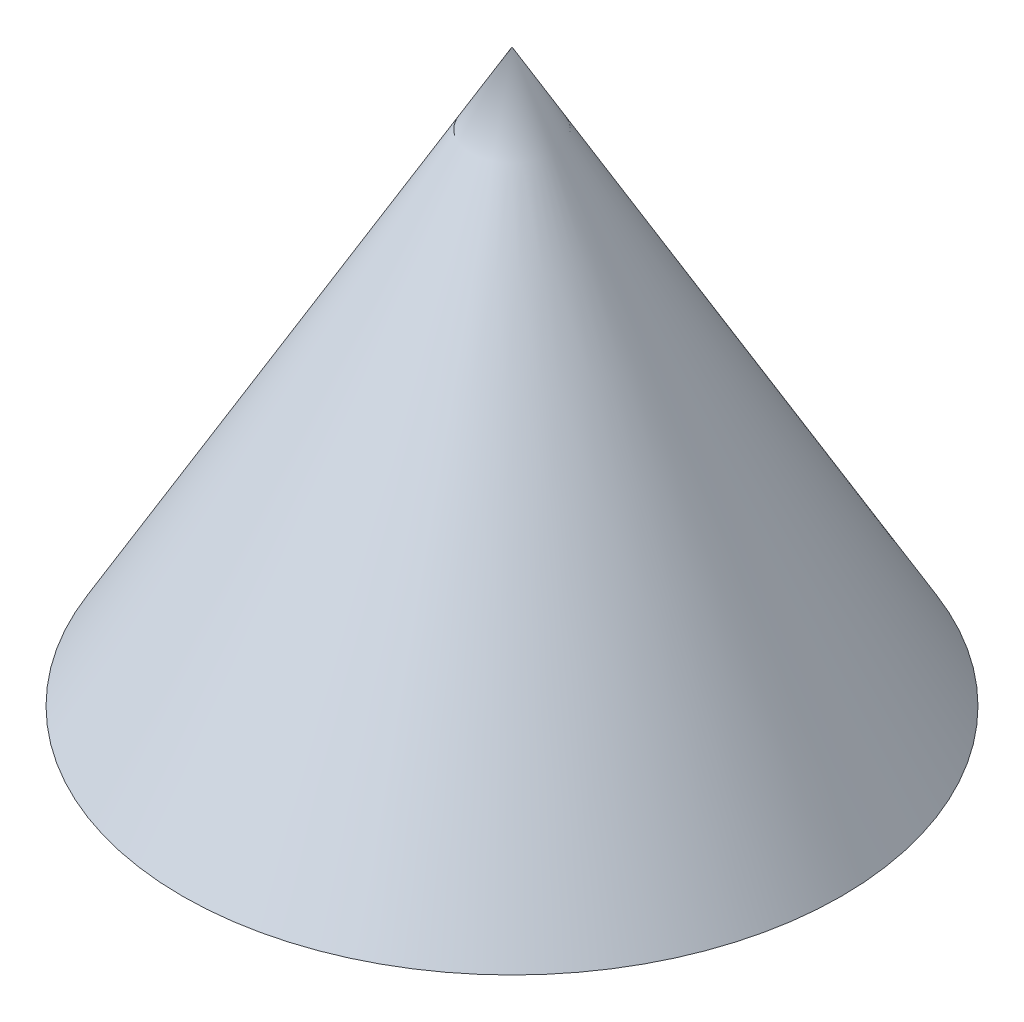
from build123d import *


with BuildPart() as part:
    # 草图1 → 旋转1 (revolve)
    with BuildSketch(Plane.XY):
        Polygon((0, 0), (57.735026919, 0), (0, 100), align=None)
    revolve(axis=Axis((0, 100, 0), (0, -1, 0)))


solid = part.part
